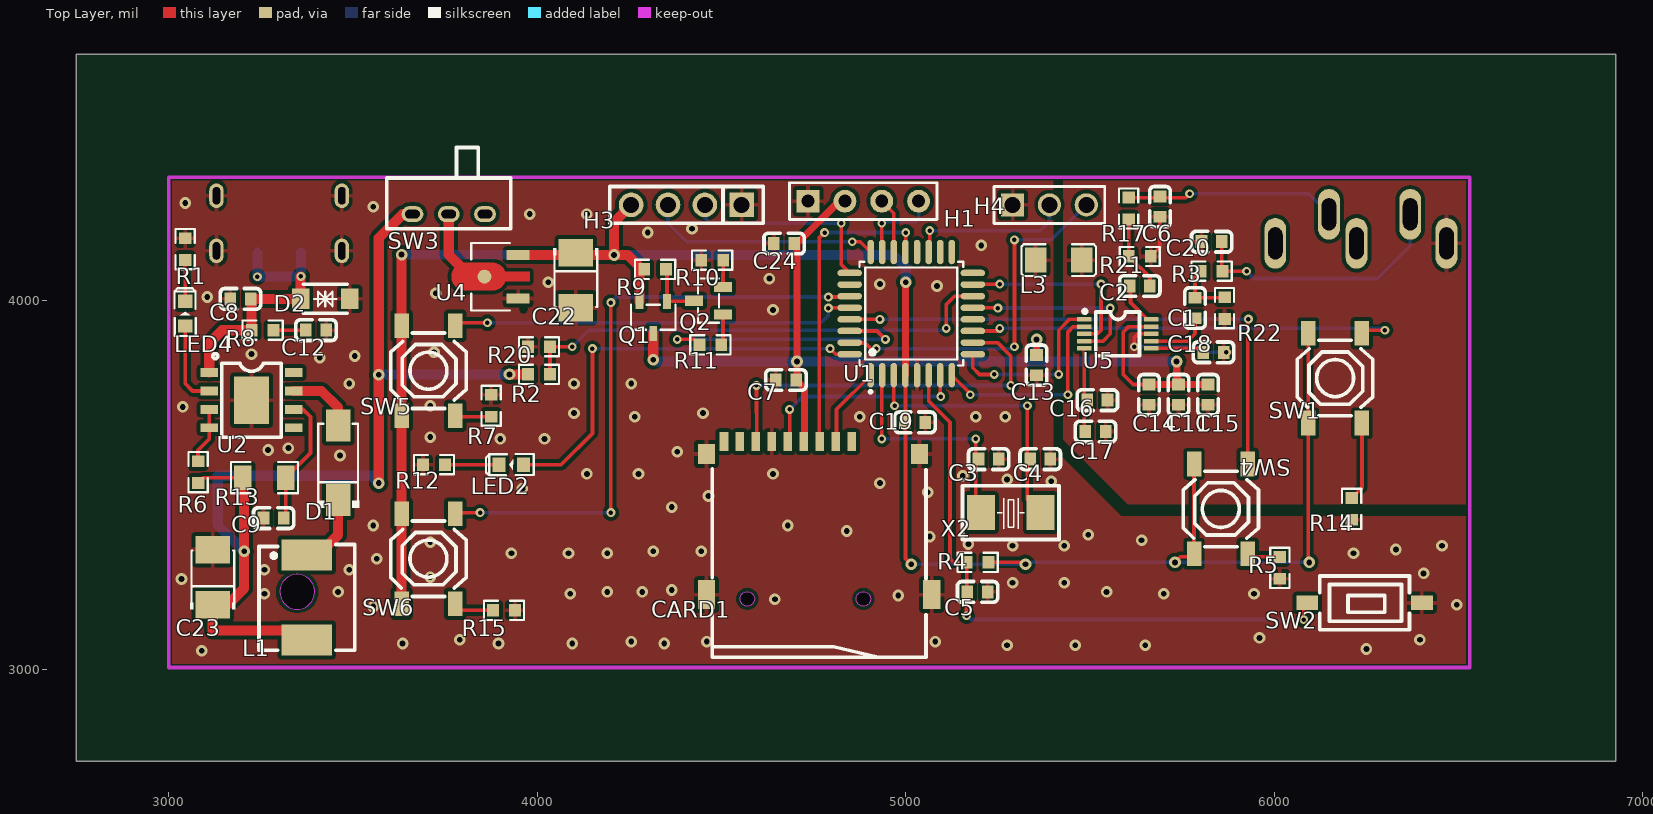
[diagram p0: Top Layer view]
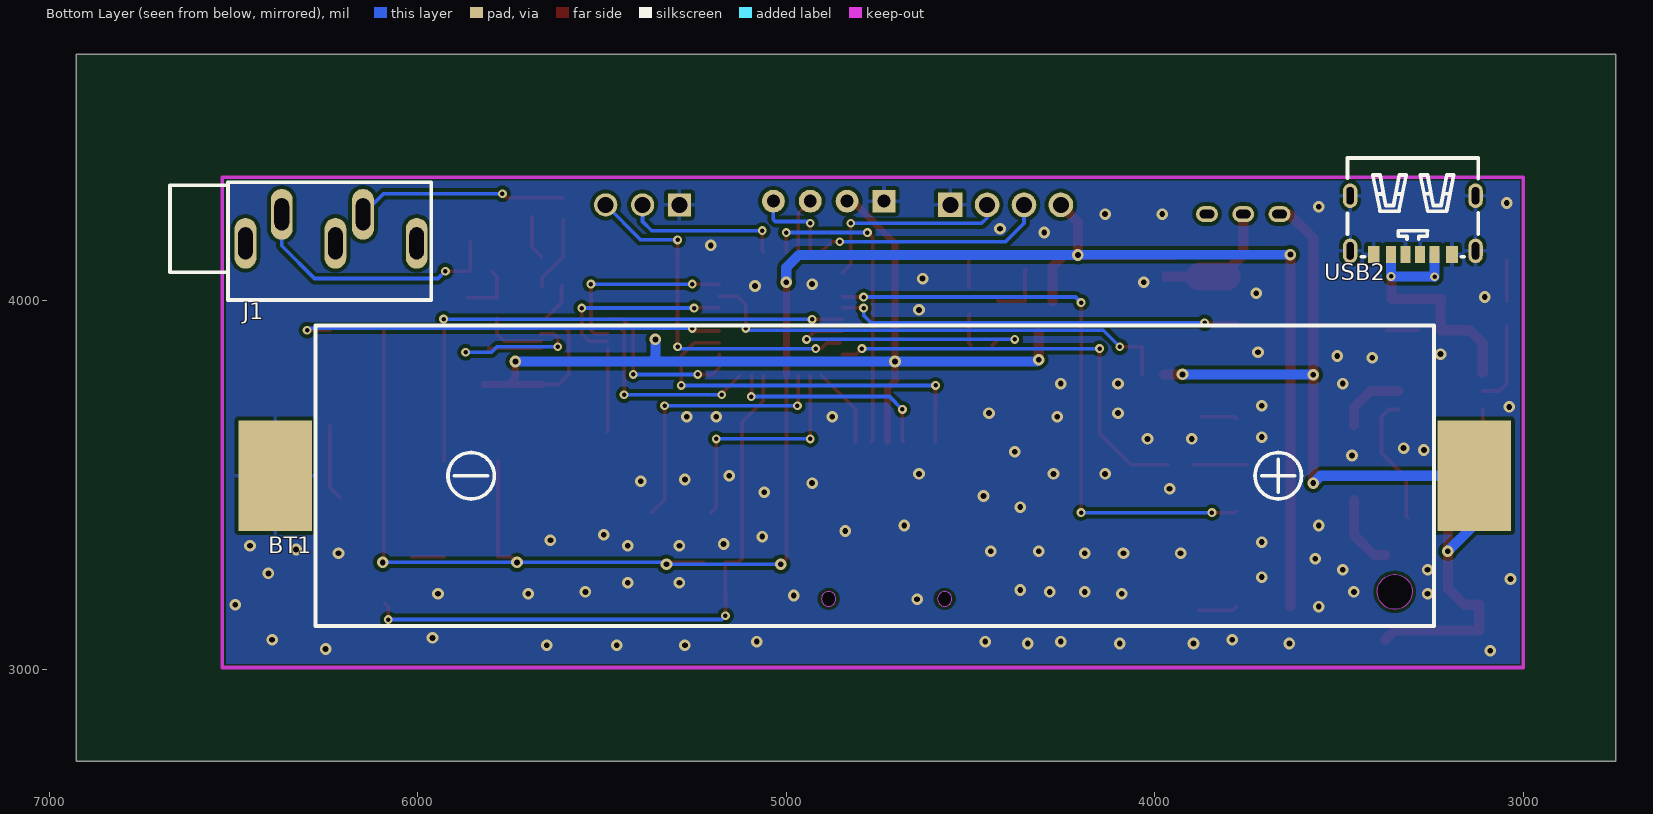
[diagram p1: Bottom Layer view, seen from below]
# Altium PCB MISC82317.pcbdoc
Units mil, origin at the board's own origin, x right, y up, seen from the top; angles counter-clockwise.
Board outline 4175.9 x 1918.1 mil, 2 copper layers (Top Layer, Bottom Layer), stack 62.2 mil thick; 67 components, 58 nets, 218 pads, 165 vias.

## Layer stack, top to bottom
Top Solder Mask Layer: solder mask 0.4, Dk 3.3
Top Layer: signal copper 1.4
Dielectric1: surface 59.4, FR4, Dk 4.5
Bottom Layer: signal copper 1.4
Bottom Solder Mask Layer: solder mask 0.4, Dk 3.3

## Board outline
6925.9,2750 2750,2750 2750,4668.1 6925.9,4668.1

## Design rules (kind name [scope] priority, off if disabled: settings)
BoardOutlineClearance copperThickness1oz [All] p0: genericclearance=10 ignorepadtopadclearanceinfootprint=FALSE except(0: Arc-SplitContinuation Track-SplitContinuation SMDPad-SplitContinuation THPad-SplitContinuation Via-SplitContinuation Fill-SplitContinuation Poly-SplitContinuation Region-SplitContinuation Text-SplitContinuation)
BoardOutlineClearance copperThickness2oz [All] p0: genericclearance=10 ignorepadtopadclearanceinfootprint=FALSE except(0: Arc-SplitContinuation Track-SplitContinuation SMDPad-SplitContinuation THPad-SplitContinuation Via-SplitContinuation Fill-SplitContinuation Poly-SplitContinuation Region-SplitContinuation Text-SplitContinuation)
BoardOutlineClearance otherClearance [All] p0: genericclearance=10 ignorepadtopadclearanceinfootprint=FALSE except(0: Arc-SplitContinuation Track-SplitContinuation SMDPad-SplitContinuation THPad-SplitContinuation Via-SplitContinuation Fill-SplitContinuation Poly-SplitContinuation Region-SplitContinuation Text-SplitContinuation)
Clearance copperThickness1oz [All] p1: gap=7 ignorepadtopadclearanceinfootprint=FALSE
Clearance copperThickness2oz [All] p1: gap=7 ignorepadtopadclearanceinfootprint=FALSE
Clearance otherClearance [All] p1: gap=7 ignorepadtopadclearanceinfootprint=FALSE
DiffPairsRouting differentialPair [All] p1: maxuncoupledlength=10 minlimit=6 maxlimit=Infinity mostfreqgap=6 toplayer_minwidth=5 toplayer_prefwidth=10 toplayer_maxwidth=100 bottomlayer_minwidth=5 bottomlayer_prefwidth=10 bottomlayer_maxwidth=100
PasteMaskExpansion pasteMaskExpansion [All] p1: expansion=0
PlaneConnect innerPlane [All] p1: planeconnectstyle=Relief reliefexpansion=20 reliefentries=4 reliefconductorwidth=10 reliefairgap=10
PolygonConnect copperRegion [All] p1: connectstyle=Relief reliefentries=4 reliefconductorwidth=10 polygonreliefangle="90 Angle" airgapwidth=10
RoutingVias viaSize [All] p1: viastyle="Through Hole" holewidth=12.0078 minholewidth=11.811 maxholewidth=248.0314 width=12.0078 minwidth=11.811 maxwidth=248.0314
SolderMaskExpansion solderMaskExpansion [IsVia] p1: useseparateexpansions=TRUE expansion=-1000 expansionbottom=-1000
SolderMaskExpansion solderMaskExpansion [All] p2: useseparateexpansions=TRUE expansion=2 expansionbottom=2
Width copperThickness1oz [All] p1: maxlimit=100 minlimit=5 preferedwidth=10
Width copperThickness2oz [All] p1: maxlimit=100 minlimit=8 preferedwidth=10

## Components (designator, comment, footprint, x,y, rotation, side; value= is the part's Value field where it differs from the comment)
BT1 "BH-18650-B1BA002" BATTERY-SMD_18650-1S-L77.1-W20.7-1 4760,3525 r270 bottom
C1 "2.2uF" C0603 5785,3980 r90 top
C2 "2.2uF" C0603 5635,4040 r0 top
C3 "20p" C0603 5225,3570 r180 top
C4 "20p" C0603 5365,3570 r180 top
C5 "10u" C0603 5195,3210 r180 top
C6 "2.2nf" C0603 5690,4255 r90 top
C7 "0.1uf" C0603 4675,3785 r0 top
C8 "22uf" C0603 3195,4005 r0 top
C9 "22uF" C0603 3285,3410 r0 top
C11 "0.1u" C0603 5740,3745 r90 top
C12 "10uF" C0603 3400,3920 r180 top
C13 "10u" C0603 5355,3825 r90 top
C14 "2.2uf" C0603 5660,3745 r90 top
C15 "10nf" C0603 5820,3745 r90 top
C16 "0.1u" C0603 5520,3730 r180 top
C17 "10u" C0603 5515,3645 r180 top
C18 "10u" C0603 5835,3860 r180 top
C19 "2.2uf" C0603 5025,3670 r180 top
C20 "2.2nf" C0603 5830,4160 r180 top
C22 "22uF" CAP-SMD_L3.5-W2.8-R-RD#1 4105,4055 r90 top
C23 "22uF" CAP-SMD_L3.5-W2.8-R-RD#2 3120,3250 r270 top
C24 "0.1uf" C0603 4670,4155 r0 top
CARD1 "TF-01A" TF-SMD_TF-01A 4765,3410 r0 top
D1 "SS14" SMA_L4.2-W2.6-LS5.3-RD 3460,3560 r90 top
D2 "SMF6.0CA" SOD-123FL_L2.8-W1.8-LS3.7-BI 3425,4005 r180 top
H1 "HDR-F-2.54_1x4" HDR-F-2.54_1X4 4885,4270 r0 top
H3 "220S-1*4P H=8.5MM" HDR-TH_4P-P2.54-V-F 4405,4260 r180 top
H4 "Z-211-0311-0021-001" HDR-TH_3P-P2.54-V-M-1 5390,4260 r0 top
J1 "PJ-325M/3.5MM" AUDIO-TH_PJ-325C 6235,4195 r180 bottom
L1 "1uH" IND-SMD_L6.8-W6.8_SMMS0630 3375,3195 r270 top
L3 "600Ω" L1206 5415,4110 r180 top
LED2 "LED-0603_G" LED0603_GREEN 3930,3555 r180 top
LED4 "LED-0603_G" LED0603_GREEN 3045,3965 r90 top
Q1 "SI2301CDS-T1-GE3" SOT-23-3_L3.0-W1.7-P0.95-LS2.9-BR 4315,3955 r90 top
Q2 "SI2302_C351401" SOT-23-3_L2.9-W1.3-P1.90-LS2.4 4465,3999.9 r0 top
R1 "10k" R0603 3045,4140 r90 top
R2 "47k" R0603 4005,3800 r180 top
R3 "470R" R0603 5830,4080 r180 top
R4 "1k" R0603 5195,3290 r0 top
R5 "10K" R0603 6015,3275 r90 top
R6 "120" R0603 3080,3535 r270 top
R7 "10K" R0603 3875,3715 r270 top
R8 "120" R0603 3255,3920 r0 top
R9 "1M" R0603 4320,4085 r0 top
R10 "100K" R0603 4475,4110 r180 top
R11 "10K" R0603 4470,3880 r0 top
R12 "10k" R0603 3720,3555 r0 top
R13 "0R5" R1206 3260,3520 r180 top
R14 "10K" R0603 6210,3435 r90 top
R15 "10K" R0603 3910,3160 r180 top
R17 "470R" R0603 5605,4250 r270 top
R20 "100k" R0603 4005,3875 r0 top
R21 "NA" R0603 5635,4120 r0 top
R22 "NA" R0603 5865,3980 r90 top
SW1 "TS-1187A-B-A-B" SW-SMD_4P-L5.1-W5.1-P3.70-LS6.5-TL-2 6165,3790 r90 top
SW2 "TS-1092S-B3D2-G" SW-SMD_L6.1-W3.6-LS7.9 6245,3180 r180 top
SW3 "MK-12D18-G020" SW-TH_MK-12D18-G040 3760,4235 r180 top
SW4 "TS-1187A-B-A-B" SW-SMD_4P-L5.1-W5.1-P3.70-LS6.5-TL-2 5855,3435 r90 top
SW5 "TS-1187A-B-A-B" SW-SMD_4P-L5.1-W5.1-P3.70-LS6.5-TL-2 3705,3810 r90 top
SW6 "TS-1187A-B-A-B" SW-SMD_4P-L5.1-W5.1-P3.70-LS6.5-TL-2 3705,3300 r90 top
U1 "STM32G070KBT6" LQFP-32_L7.0-W7.0-P0.80-LS9.0-BL 5015,3965 r0 top
U2 "IP5306" ESOP-8_L4.9-W3.9-P1.27-LS6.0-BL-EP 3225,3730 r270 top
U4 "HT7833" SOT-89_L4.5-W2.5-P1.50-LS4.2-BR 3895,4065 r0 top
U5 "CS4344" TSSOP-10_L3.0-W3.0-P0.50-LS4.9-BL 5575,3910 r270 top
USB2 "TYPE-C 6P" TYPE-C-SMD_TYPE-C-6P 3300,4205 r0 bottom
X2 "8MHz" CRYSTAL-SMD_L5.0-W3.2 5285,3425 r0 top

## Footprints (in the part's own frame and the unit in brackets; to place one, negate y for a bottom-side part, rotate by r counter-clockwise, add the part's x,y. Pads: shape width x height; smd on the part's side, far side on the other; paste and mask are expansions set on the pad)
AUDIO-TH_PJ-325C [mil]
  oval 59.1x137.8 hole 39.4 slot 86.6 at 90 deg: 1(-232.3,-39.4) 2(11.8,-39.4) 3(86.6,39.4) 4(232.3,-39.4) 5(-133.9,39.4)
  silkscreen extent -437,-193 272,126
BATTERY-SMD_18650-1S-L77.1-W20.7-1 [mil]
  rect 300x200 smd: 1(0,-1626.5) 2(0,1626.5)
  Board Outline Layer lines w0.1: 316.5,1458.2 310.4,1458 304.4,1457.1 298.6,1455.4 293.1,1452.9 287.9,1449.8 283.2,1446 279,1441.6 275.4,1436.8 272.4,1431.5 270.1,1425.9 268.6,1420.1 267.8,1414 267.8,1408 268.6,1402 270.1,1396.1 272.4,1390.5 275.4,1385.2 279,1380.4 283.2,1376 287.9,1372.3 293.1,1369.1 298.6,1366.7 304.4,1365 310.4,1364 316.5,1363.8 322.5,1364.4 328.4,1365.7 334.1,1367.8 339.5,1370.6 344.4,1374.1 348.9,1378.2 352.8,1382.8 356.1,1387.8 358.8,1393.3 360.7,1399 361.8,1405 362.2,1411 361.8,1417.1 360.7,1423 358.8,1428.7 356.1,1434.2 352.8,1439.3 348.9,1443.9 344.4,1448 339.5,1451.4 334.1,1454.2 328.4,1456.3 322.5,1457.7 316.5,1458.2
  Board Outline Layer region: 362.2,1411 361.8,1405 360.7,1399 358.8,1393.3 356.1,1387.8 352.8,1382.8 348.9,1378.2 344.4,1374.1 339.5,1370.6 334.1,1367.8 328.4,1365.7 322.5,1364.4 316.5,1363.8 310.4,1364 304.4,1365 298.6,1366.7 293.1,1369.1 287.9,1372.3 283.2,1376 279,1380.4 275.4,1385.2 272.4,1390.5 270.1,1396.1 268.6,1402 267.8,1408 267.8,1414 268.6,1420.1 270.1,1425.9 272.4,1431.5 275.4,1436.8 279,1441.6 283.2,1446 287.9,1449.8 293.1,1452.9 298.6,1455.4 304.4,1457.1 310.4,1458 316.5,1458.2 322.5,1457.7 328.4,1456.3 334.1,1454.2 339.5,1451.4 344.4,1448 348.9,1443.9 352.8,1439.3 356.1,1434.2 358.8,1428.7 360.7,1423 361.8,1417.1
  Board Outline Layer region: 362.2,1411 361.8,1405 360.7,1399 358.8,1393.3 356.1,1387.8 352.8,1382.8 348.9,1378.2 344.4,1374.1 339.5,1370.6 334.1,1367.8 328.4,1365.7 322.5,1364.4 316.5,1363.8 310.4,1364 304.4,1365 298.6,1366.7 293.1,1369.1 287.9,1372.3 283.2,1376 279,1380.4 275.4,1385.2 272.4,1390.5 270.1,1396.1 268.6,1402 267.8,1408 267.8,1414 268.6,1420.1 270.1,1425.9 272.4,1431.5 275.4,1436.8 279,1441.6 283.2,1446 287.9,1449.8 293.1,1452.9 298.6,1455.4 304.4,1457.1 310.4,1458 316.5,1458.2 322.5,1457.7 328.4,1456.3 334.1,1454.2 339.5,1451.4 344.4,1448 348.9,1443.9 352.8,1439.3 356.1,1434.2 358.8,1428.7 360.7,1423 361.8,1417.1
  Multi-Layer board cut-out: 362.2,1411 361.8,1405 360.7,1399 358.8,1393.3 356.1,1387.8 352.8,1382.8 348.9,1378.2 344.4,1374.1 339.5,1370.6 334.1,1367.8 328.4,1365.7 322.5,1364.4 316.5,1363.8 310.4,1364 304.4,1365 298.6,1366.7 293.1,1369.1 287.9,1372.3 283.2,1376 279,1380.4 275.4,1385.2 272.4,1390.5 270.1,1396.1 268.6,1402 267.8,1408 267.8,1414 268.6,1420.1 270.1,1425.9 272.4,1431.5 275.4,1436.8 279,1441.6 283.2,1446 287.9,1449.8 293.1,1452.9 298.6,1455.4 304.4,1457.1 310.4,1458 316.5,1458.2 322.5,1457.7 328.4,1456.3 334.1,1454.2 339.5,1451.4 344.4,1448 348.9,1443.9 352.8,1439.3 356.1,1434.2 358.8,1428.7 360.7,1423 361.8,1417.1
  silkscreen extent -408,-1518 408,1518
C0603 [mil]
  rect 31.5x35.4 smd: 1(-27.6,0) 2(27.6,0)
  silkscreen extent -55,-28 55,28
CAP-SMD_L3.5-W2.8-R-RD#1 [mil]
  rect 74.8x93.5 smd: 1(74.8,0) 2(-74.7,0)
  silkscreen extent -72,-61 87,61
CAP-SMD_L3.5-W2.8-R-RD#2 [mil]
  rect 74.8x93.5 smd: 1(74.7,0) 2(-74.8,0)
  silkscreen extent -72,-61 87,61
CRYSTAL-SMD_L5.0-W3.2 [mil]
  rect 74.8x94.5 smd: 1(-80.7,0) 2(80.7,0)
  silkscreen extent -131,-73 131,73
ESOP-8_L4.9-W3.9-P1.27-LS6.0-BL-EP [mil]
  rect 23.6x47.2 smd: 1(-75,-114.5) 2(-25,-114.5) 3(25,-114.5) 4(75,-114.5) 5(75,114.5) 6(25,114.5) 7(-25,114.5) 8(-75,114.5)
  rect 129.9x94.5 smd: 9(0,0)
  silkscreen extent -126,-105 100,81
HDR-F-2.54_1X4 [mil]
  rect 62x62 hole 35: 1(-150,0)
  round 62 hole 35: 2(-50,0) 3(50,0) 4(150,0)
  silkscreen extent -200,-50 200,50
HDR-TH_3P-P2.54-V-M-1 [mil]
  rect 62x63 hole 43.3 paste+0 mask+2: 1(-100,0)
  round 63 hole 43.3 paste+0 mask+2: 2(0,0) 3(100,0)
  silkscreen extent -150,-50 150,50
HDR-TH_4P-P2.54-V-F [mil]
  rect 66.9x66.9 hole 43.3: 1(-150,0)
  round 66.9 hole 43.3: 2(-50,0) 3(50,0) 4(150,0)
  silkscreen extent -208,-50 208,50
IND-SMD_L6.8-W6.8_SMMS0630 [mil]
  rect 84.6x137.8 smd paste+0 mask+2: 1(-115.2,0) 2(115.2,0)
  silkscreen extent -144,-130 144,130
L1206 [mil]
  rect 58.5x68 smd paste-3937 mask+2: 1(-62.7,0) 2(62.7,0)
  silkscreen extent -101,-43 101,43
LED0603_GREEN [mil]
  rect 35.4x39.4 smd: 1(-33.5,0) 2(33.5,0)
  silkscreen extent -61,-29 69,29
LQFP-32_L7.0-W7.0-P0.80-LS9.0-BL [mil]
  oval 17.6x66.3 smd: 1(-110.2,-167) 2(-78.7,-167) 3(-47.2,-167) 4(-15.7,-167) 5(15.8,-167) 6(47.2,-167) 7(78.7,-167) 8(110.2,-167) 17(110.2,167) 18(78.7,167) 19(47.2,167) 20(15.8,167) 21(-15.7,167) 22(-47.2,167) 23(-78.7,167) 24(-110.2,167)
  oval 66.3x17.6 smd: 9(167,-110.2) 10(167,-78.7) 11(167,-47.2) 12(167,-15.7) 13(167,15.8) 14(167,47.2) 15(167,78.7) 16(167,110.2) 25(-167,110.2) 26(-167,78.7) 27(-167,47.2) 28(-167,15.8) 29(-167,-15.7) 30(-167,-47.2) 31(-167,-78.7) 32(-167,-110.2)
  silkscreen extent -141,-216 141,141
R0603 [mil]
  rect 31.8x34 smd paste-3937 mask+2: 1(-29.7,0) 2(29.7,0)
  silkscreen extent -54,-26 54,26
R1206 [mil]
  rect 47.5x67 smd paste-3937 mask+2: 1(-58.2,0) 2(58.2,0)
  silkscreen extent -91,-43 91,43
SMA_L4.2-W2.6-LS5.3-RD [mil]
  rect 86.6x66.9 smd: 1(-101,0) 2(101,0)
  silkscreen extent -121,-57 106,57
SOD-123FL_L2.8-W1.8-LS3.7-BI [mil]
  rect 47.2x55.1 smd: 1(-66.9,0) 2(66.9,0)
  silkscreen extent -59,-39 59,39
SOT-23-3_L2.9-W1.3-P1.90-LS2.4 [mil]
  rect 49.2x27.6 smd: 1(39.4,-37.4) 2(39.4,37.4) 3(-39.3,0)
  silkscreen extent -28,-60 29,60
SOT-23-3_L3.0-W1.7-P0.95-LS2.9-BR [mil]
  rect 40.8x20.9 smd: 1(43.4,-37.4) 2(43.4,37.4) 3(-43.4,0)
  silkscreen extent -34,-60 34,60
SOT-89_L4.5-W2.5-P1.50-LS4.2-BR [mil]
  rect 62x26.5 smd paste+0 mask+2: 1(53.4,-59.1) 3(53.4,59.1)
  round 37.4 smd: 2(-38,0.3)
  Top Layer region: -89.9,37.7 -16.9,37.7 -15.1,37.7 -13.4,37.6 -11.6,37.4 -9.9,37.1 -8.2,36.7 -6.5,36.3 -4.8,35.7 -3.2,35.1 -1.6,34.5 0,33.7 1.6,32.9 3.1,32 4.5,31 5.9,30 7.3,28.9 8.6,27.7 9.9,26.5 11.1,25.2 12.2,23.9 13.3,22.5 14.3,21 15.2,19.5 16.1,18 16.9,16.5 17.6,13.3 84.4,13.3 84.4,-12.6 17.6,-12.6 16.9,-15.8 16.1,-17.3 15.2,-18.9 14.3,-20.3 13.3,-21.8 12.2,-23.2 11.1,-24.5 9.9,-25.8 8.6,-27 7.3,-28.2 5.9,-29.3 4.5,-30.3 3.1,-31.3 1.6,-32.2 0,-33 -1.6,-33.8 -3.2,-34.5 -4.8,-35.1 -6.5,-35.6 -8.2,-36 -9.9,-36.4 -11.6,-36.7 -13.4,-36.9 -15.1,-37 -16.9,-37.1 -89.9,-37.1 -91.6,-37 -93.4,-36.9 -95.1,-36.7 -96.9,-36.4 -98.6,-36 -100.3,-35.6 -101.9,-35.1 -103.6,-34.5 -105.2,-33.8 -106.8,-33 -108.3,-32.2 -109.8,-31.3 -111.3,-30.3 -112.7,-29.3 -114.1,-28.2 -115.4,-27 -116.6,-25.8 -117.8,-24.5 -119,-23.2 -120,-21.8 -121.1,-20.3 -122,-18.9 -122.8,-17.3 -123.6,-15.8 -124.4,-14.2 -125,-12.5 -125.6,-10.9 -126.1,-9.2 -126.5,-7.5 -126.8,-5.8 -127,-4 -127.2,-2.3 -127.3,-0.5 -127.3,1.2 -127.2,3 -127,4.7 -126.8,6.5 -126.5,8.2 -126.1,9.9 -125.6,11.6 -125,13.2 -124.4,14.9 -123.6,16.5 -122.8,18 -122,19.5 -121.1,21 -120,22.5 -119,23.9 -117.8,25.2 -116.6,26.5 -115.4,27.7 -114.1,28.9 -112.7,30 -111.3,31 -109.8,32 -108.3,32.9 -106.8,33.7 -105.2,34.5 -103.6,35.1 -101.9,35.7 -100.3,36.3 -98.6,36.7 -96.9,37.1 -95.1,37.4 -93.4,37.6 -91.6,37.7
  silkscreen extent -74,-92 31,92
SW-SMD_4P-L5.1-W5.1-P3.70-LS6.5-TL-2 [mil]
  rect 66.9x39.4 smd: 1(-122,72.8) 2(122,72.8) 3(-122,-72.8) 4(122,-72.8)
  silkscreen extent -102,-102 102,102
SW-SMD_L6.1-W3.6-LS7.9 [mil]
  rect 59.1x39.4 smd: 1(-155.5,0) 2(155.5,0)
  silkscreen extent -122,-73 122,73
SW-TH_MK-12D18-G040 [mil]
  oval 59.1x43.3 hole 23.6 slot 39.4 at 0 deg paste+0 mask+2: 1(-98.4,0) 2(0,0) 3(98.4,0)
  silkscreen extent -168,-181 168,40
TF-SMD_TF-01A [mil]
  rect 23.6x51.2 smd: 1(88.2,207.7) 2(44.9,207.7) 3(1.6,207.7) 4(-41.7,207.7) 5(-85,207.7) 6(-128.3,207.7) 7(-171.7,207.7) 8(-215,207.7) 9(-258.3,207.7)
  rect 47.2x55.1 smd: 10(-305.5,174.2) 13(272.4,174.2)
  rect 47.2x78.7 smd: 11(-305.5,-207.7) 12(305.5,-207.7)
  Board Outline Layer lines w0.1: -214.6,-219.1 -214.2,-223 -213.1,-226.7 -211.2,-230.1 -208.8,-233.1 -205.8,-235.5 -202.4,-237.3 -198.7,-238.4 -194.9,-238.8 -191,-238.4 -187.3,-237.3 -183.9,-235.5 -181,-233.1 -178.5,-230.1 -176.7,-226.7 -175.6,-223 -175.2,-219.1 -175.6,-215.3 -176.7,-211.6 -178.5,-208.2 -181,-205.2 -183.9,-202.8 -187.3,-201 -191,-199.8 -194.9,-199.5 -198.7,-199.8 -202.4,-201 -205.8,-202.8 -208.8,-205.2 -211.2,-208.2 -213.1,-211.6 -214.2,-215.3 -214.6,-219.1 ; 100.4,-219.1 100.8,-223 101.9,-226.7 103.7,-230.1 106.2,-233.1 109.1,-235.5 112.5,-237.3 116.2,-238.4 120.1,-238.8 123.9,-238.4 127.6,-237.3 131,-235.5 134,-233.1 136.4,-230.1 138.3,-226.7 139.4,-223 139.8,-219.1 139.4,-215.3 138.3,-211.6 136.4,-208.2 134,-205.2 131,-202.8 127.6,-201 123.9,-199.8 120.1,-199.5 116.2,-199.8 112.5,-201 109.1,-202.8 106.2,-205.2 103.7,-208.2 101.9,-211.6 100.8,-215.3 100.4,-219.1
  Board Outline Layer region: -175.2,-219.1 -175.6,-223 -176.7,-226.7 -178.5,-230.1 -181,-233.1 -183.9,-235.5 -187.3,-237.3 -191,-238.4 -194.9,-238.8 -198.7,-238.4 -202.4,-237.3 -205.8,-235.5 -208.8,-233.1 -211.2,-230.1 -213.1,-226.7 -214.2,-223 -214.6,-219.1 -214.2,-215.3 -213.1,-211.6 -211.2,-208.2 -208.8,-205.2 -205.8,-202.8 -202.4,-201 -198.7,-199.8 -194.9,-199.5 -191,-199.8 -187.3,-201 -183.9,-202.8 -181,-205.2 -178.5,-208.2 -176.7,-211.6 -175.6,-215.3
  Board Outline Layer region: -175.2,-219.1 -175.6,-223 -176.7,-226.7 -178.5,-230.1 -181,-233.1 -183.9,-235.5 -187.3,-237.3 -191,-238.4 -194.9,-238.8 -198.7,-238.4 -202.4,-237.3 -205.8,-235.5 -208.8,-233.1 -211.2,-230.1 -213.1,-226.7 -214.2,-223 -214.6,-219.1 -214.2,-215.3 -213.1,-211.6 -211.2,-208.2 -208.8,-205.2 -205.8,-202.8 -202.4,-201 -198.7,-199.8 -194.9,-199.5 -191,-199.8 -187.3,-201 -183.9,-202.8 -181,-205.2 -178.5,-208.2 -176.7,-211.6 -175.6,-215.3
  Board Outline Layer region: 139.8,-219.1 139.4,-223 138.3,-226.7 136.4,-230.1 134,-233.1 131,-235.5 127.6,-237.3 123.9,-238.4 120.1,-238.8 116.2,-238.4 112.5,-237.3 109.1,-235.5 106.2,-233.1 103.7,-230.1 101.9,-226.7 100.8,-223 100.4,-219.1 100.8,-215.3 101.9,-211.6 103.7,-208.2 106.2,-205.2 109.1,-202.8 112.5,-201 116.2,-199.8 120.1,-199.5 123.9,-199.8 127.6,-201 131,-202.8 134,-205.2 136.4,-208.2 138.3,-211.6 139.4,-215.3
  Board Outline Layer region: 139.8,-219.1 139.4,-223 138.3,-226.7 136.4,-230.1 134,-233.1 131,-235.5 127.6,-237.3 123.9,-238.4 120.1,-238.8 116.2,-238.4 112.5,-237.3 109.1,-235.5 106.2,-233.1 103.7,-230.1 101.9,-226.7 100.8,-223 100.4,-219.1 100.8,-215.3 101.9,-211.6 103.7,-208.2 106.2,-205.2 109.1,-202.8 112.5,-201 116.2,-199.8 120.1,-199.5 123.9,-199.8 127.6,-201 131,-202.8 134,-205.2 136.4,-208.2 138.3,-211.6 139.4,-215.3
  Multi-Layer board cut-out: -175.2,-219.1 -175.6,-223 -176.7,-226.7 -178.5,-230.1 -181,-233.1 -183.9,-235.5 -187.3,-237.3 -191,-238.4 -194.9,-238.8 -198.7,-238.4 -202.4,-237.3 -205.8,-235.5 -208.8,-233.1 -211.2,-230.1 -213.1,-226.7 -214.2,-223 -214.6,-219.1 -214.2,-215.3 -213.1,-211.6 -211.2,-208.2 -208.8,-205.2 -205.8,-202.8 -202.4,-201 -198.7,-199.8 -194.9,-199.5 -191,-199.8 -187.3,-201 -183.9,-202.8 -181,-205.2 -178.5,-208.2 -176.7,-211.6 -175.6,-215.3
  Multi-Layer board cut-out: 139.8,-219.1 139.4,-223 138.3,-226.7 136.4,-230.1 134,-233.1 131,-235.5 127.6,-237.3 123.9,-238.4 120.1,-238.8 116.2,-238.4 112.5,-237.3 109.1,-235.5 106.2,-233.1 103.7,-230.1 101.9,-226.7 100.8,-223 100.4,-219.1 100.8,-215.3 101.9,-211.6 103.7,-208.2 106.2,-205.2 109.1,-202.8 112.5,-201 116.2,-199.8 120.1,-199.5 123.9,-199.8 127.6,-201 131,-202.8 134,-205.2 136.4,-208.2 138.3,-211.6 139.4,-215.3
  silkscreen extent -290,-377 290,134
TSSOP-10_L3.0-W3.0-P0.50-LS4.9-BL [mil]
  rect 11.8x39.4 smd: 1(-39.4,-90.6) 2(-19.7,-90.6) 3(0,-90.6) 4(19.7,-90.6) 5(39.4,-90.6) 6(39.4,90.6) 7(19.7,90.6) 8(0,90.6) 9(-19.7,90.6) 10(-39.4,90.6)
  silkscreen extent -66,-94 59,59
TYPE-C-SMD_TYPE-C-6P [mil]
  oval 39.4x66.9 hole 19.7 slot 47.2 at 90 deg paste+0 mask+2: 7(-170.1,-79.7) 7(-170.1,69.9) 7(170.1,-79.7) 7(170.1,69.9)
  rect 27.6x47.2 smd paste+0 mask+2: A5(-19.7,79.7) A9(59,79.7) B5(19.7,79.7) B9(-59.1,79.7)
  rect 31.5x47.2 smd paste+0 mask+2: A12(106.3,79.7) B12(-106.3,79.7)
  silkscreen extent -177,-182 177,86

## Via types
v1: diameter 31.5, hole 15.7, Top Layer to Bottom Layer, 116 vias
v2: diameter 24, hole 12.2, Top Layer to Bottom Layer, 47 vias
v3: diameter 24, hole 12, Top Layer to Bottom Layer, 2 vias

## Nets (pads, with @x,y where several pads share a name; then routed paths per layer and width w, separated by ;. In a path a pad name is that pad's centre, name@x,y a point inside that pad or via, vN(x,y) a via of type N, cw(c..) or ccw(c..) an arc to the next point about the centre after c; other vN are vias at no path point)
$1N1: R15.2 SW6.3 | length 106.7
  Top Layer w10: SW6.3@3777.8,3170.1 3787.9,3160 R15.2
$1N3: R7.2 SW5.3 | length 99.3
  Top Layer w10: SW5.3@3777.8,3680.1 3783.1,3685.3 R7.2
$1N5: R5.2 SW4.3 | length 87.1
  Top Layer w10: SW4.3@5927.9,3305.1 R5.2
$1N10: LED4.2 R1.1 | length 111.8
  Top Layer w10: LED4.2 R1.1
$1N24: R14.2 SW1.3 | length 207
  Top Layer w10: R14.2 6237.9,3492.5 SW1.3@6237.9,3660.1
$1N27: LED2.2 R12.2 | length 146.8
  Top Layer w10: R12.2 LED2.2
$1N29: Q2.2 R10.1 | length 72.6
  Top Layer w10: Q2.2@4504.4,4037.4 R10.1
$1N30: Q2.1 R11.2 | length 84.5
  Top Layer w10: R11.2 4504.4,3884.8 Q2.1@4504.4,3962.6
$1N54: C12.2 R8.2 | length 87.7
  Top Layer w10: R8.2 C12.2
$1N57: D1.1 L1.1 | length 201.7
  Top Layer w27.6: L1.1 3405.2,3310.2 3460,3365 D1.1
$1N70: C1.2 R3.2 R22.2 | length 159.6
  Top Layer w10: R3.2 5785,4064.7 C1.2 5862.9,4007.6 R22.2
$1N71: C2.2 R17.2 R21.1 | length 204.2
  Top Layer w10: R17.2 5605.3,4220 R21.1 5662.6,4062.8 C2.2
$1N81: C18.2 U5.6 | length 152.4
  Top Layer w10: U5.6 5807.4,3870.6 C18.2
$1N104: C16.2 C17.2 U5.5 | length 226.8
  Top Layer w10: U5.5 5484.4,3648 C17.2
$1N113: Q1.1 Q2.3 R9.2 | length 161.6
  Top Layer w10: R9.2 4352.4,4082.3 Q1.1 4424.1,3998.4 Q2.3
$1N116: C9.2 R13.1 U2.6 | length 358.7
  Top Layer w10: C9.2 3318.2,3415.7 R13.1 3385,3586.8 3385,3685 3365,3705 U2.6
$1N117: D1.2 U2.7 | length 188.1
  Top Layer w27.6: U2.7 3415,3755 3460,3710 D1.2
$1N119: R6.1 U2.3 U2.4 | length 152.9
  Top Layer w10: R6.1 3080,3594.5 3110.5,3625 U2.4 U2.3
$1N120: SW3.2 U4.2 | length 216.3
  Top Layer w27.6: SW3.2 3760,4125 3819.7,4065.3 U4.2@3841.6,4065.3
$1N123: LED4.1 U2.2 | length 230.3
  Top Layer w10: LED4.1 3045,3775 3065,3755 U2.2
$1N128: C6.2 J1.3 R17.1 | length 570.7
  Top Layer w10: R17.1 5759.7,4279.7 v2(5770,4290)
  Bottom Layer w10: v2(5770,4290) 6092.8,4290 J1.3
$1N129: C20.1 J1.5 R3.1 | length 720.7
  Top Layer w10: C20.1 5857.6,4082.1 R3.1 v2(5925,4080)
  Bottom Layer w10: v2(5925,4080) 5945,4060 6280,4060 6368.9,4148.9 J1.5
A-GND: C6.1 C11.1 C14.1 C15.1 C16.1 C17.1 C18.1 C20.2 J1.1 L3.1 R21.2 R22.1 U5.8 | length 448.8
  Top Layer w10: v3(5620,3875) 5620,3900 5630,3910 U5.8 ; R21.2 5690,4145.3 C6.1
  Bottom Layer w10: v3(5620,3875) 5785,3875 5800,3860 v3(5870,3860)
AUDIO-L: C1.1 U5.7 | length 170
  Top Layer w10: U5.7 5765.3,3890.3 5785,3910 C1.1
AUDIO-R: C2.1 U5.10 | length 120.6
  Top Layer w10: C2.1 5610,4037.4 5610,3995 5655.6,3949.4 U5.10
BADC: R2.1 R20.2 U1.14 | length 1327.2
  Top Layer w10: R2.1 R20.2 v2(4095,3875) ; v2@5115,3920 v2(5110,3925) 5110,3990 5132.2,4012.2 U1.14
  Bottom Layer w10: v2(4095,3875) 4140,3920 5110,3920 v2(5110,3925)
GND: BT1.1 C3.1 C4.1 C5.1 C7.1 C8.1 C9.1 C12.1 C13.1 C19.1 C22.2 C23.2 C24.1 CARD1.6 CARD1.10 CARD1.11 CARD1.12 CARD1.13 D2.1 H1.1 H3.1 H4.1 L3.2 R1.2 R5.1 R7.1 R10.2 R12.1 R14.1 R15.1 R20.1 SW2.1 U1.5 U2.9 U4.1 USB2.7 USB2.A5 USB2.A12 USB2.B5 USB2.B12
  other v1: 3090,3050 6250,3055 5275,3065 5460,3065 5650,3065 3635,3070 3895,3070 4095,3070 4345,3070 4255,3075 4460,3075 5080,3075 3790,3080 6395,3080 5960,3085 3555,3170 6495,3175 4645,3190 4980,3200 3260,3205 4090,3205 5700,3205 5945,3205 3460,3210 4190,3210 4285,3210 5545,3210 4365,3215 5290,3235 5430,3235 3035,3245 3710,3250 6405,3260 3260,3270 3490,3270 3565,3300 3930,3315 4085,3315 4190,3315 6215,3315 4315,3320 4445,3320 6330,3325 5290,3335 5430,3335 6455,3335 5170,3340 3710,3345 5640,3350 5065,3360 5495,3365 4840,3375 3555,3390 4680,3390 4365,3440 4465,3470 5060,3480 3960,3490 4930,3505 5395,3510 5275,3515 5155,3525 4135,3530 4275,3530 4640,3530 3465,3580 4380,3590 3270,3595 3325,3600 3900,3625 4020,3625 3710,3630 4265,3685 4875,3685 5190,3685 5270,3685 4100,3695 4450,3695 3038.3,3711.8 3710,3715 3490,3775 4100,3775 4255,3775 3410,3845 3505,3850 3225,3855 3720,3860 4640,3975 3105,4010 3725,4020 5085,4040 4930,4045 4030,4050 4630,4060 5205,4150 4300,4185 4420,4195 3980,4235 4135,4235 3555,4255 3045,4265
I2S-CLK: U1.8 U5.2 | length 559.2
  Top Layer w10: U1.8 5175,3748.2 v2(5175,3745) ; v2(5440,3745) 5440,3915 5454.7,3929.7 U5.2@5484.5,3929.7
  Bottom Layer w10: v2(5175,3745) v2(5440,3745)
I2S-MCLK: U1.13 U5.4 | length 521.8
  Top Layer w10: U1.13@5182,3980.7 v2(5250,3980) ; U5.4 5535.3,3890.3 5555,3910 v2(5555,3980)
  Bottom Layer w10: v2(5250,3980) v2(5555,3980)
I2S-SDIN: U1.9 U5.1 | length 478.9
  Top Layer w10: U1.9 5182,3818 5200,3800 v2(5240,3800) ; v2(5415,3800) 5415,3920 5444.4,3949.4 U5.1@5484.5,3949.4
  Bottom Layer w10: v2(5240,3800) v2(5415,3800)
I2S-WS: U1.15 U5.3 | length 523.2
  Top Layer w10: U1.15 5183.3,4045 v2(5255,4045) ; U5.3@5484.5,3910 5520,3910 5530,3920 v2(5530,4045)
  Bottom Layer w10: v2(5255,4045) v2(5530,4045)
KEY-2:  | length 1468.2
  Top Layer w10: 4848,3949.3 v2(4930,3949.3) ; 5927.9,3564.9 5927.9,3947.8 v2(5930,3950)
  Bottom Layer w10: v2(4930,3949.3) 5929.3,3949.3 v2(5930,3950)
Key-2: SW4.4 U1.29
KEY-3:  | length 1098.5
  Top Layer w10: 3777.8,3939.9 v2(3865,3940) ; v2(4790,3980) 4848,3980.7
  Bottom Layer w10: v2(3865,3940) 4770,3940 4790,3960 v2(4790,3980)
Key-3: SW5.4 U1.28
KEY-4:  | length 1649.3
  Top Layer w10: 3777.8,3429.9 3782.8,3425 v2(3845,3425) ; v2(4200,3425) v2(4200,3995) ; v2(4790,4010) 4845.8,4010 4848,4012.2
  Bottom Layer w10: v2(3845,3425) v2(4200,3425) ; v2(4200,3995) 4215,4010 v2(4790,4010)
Key-4: SW6.4 U1.27
KEY-WAKE:  | length 1185.2
  Top Layer w10: 5182,3917.8 5247.8,3917.8 v2(5255,3925) ; 6237.9,3919.9 v2(6300,3920)
  Bottom Layer w10: v2(5255,3925) 6295,3925 v2(6300,3920)
Key-Wake: SW1.4 U1.11
NRST: C5.2 R4.1 SW2.2 U1.6 | length 1686.3
  Top Layer w10: U1.6 5062.2,3727.8 5120,3670 5120,3300 5130,3290 R4.1 5165.3,3212.1 C5.2 5165,3207.6 v2(5165,3145) ; v2(6080,3135) 6080,3170.5 SW2.2
  Bottom Layer w10: v2(5165,3145) 5175,3135 v2(6080,3135)
PERI-CNT: R11.1 U1.30 | length 738
  Top Layer w10: v2(4380,3895) 4425.3,3895 R11.1 ; U1.30 4922.2,3917.8 v2(4945,3895)
  Bottom Layer w10: v2(4380,3895) v2(4945,3895)
SCL: H1.3 U1.22 | length 151.6
  Top Layer w10: H1.3 4967.8,4237.2 U1.22
SDA: H1.4 U1.23 | length 235.6
  Top Layer w10: v2(4935,4210) 4935,4133.3 U1.23
  Bottom Layer w10: v2(4935,4210) 4935,4215 5030,4215 5035,4220 H1.4
SPI-CS: CARD1.2 U1.1 | length 218.6
  Top Layer w10: CARD1.2@4812.3,3617.7 4812.3,3705.5 U1.1
SPI-MISO: CARD1.7 U1.10 | length 1040.3
  Top Layer w10: v2(4595,3770) CARD1.7@4595.7,3617.7 ; U1.10 5248.7,3886.3 5285,3850 v2(5285,3770)
  Bottom Layer w10: v2(4595,3770) v2(5285,3770)
SPI-MOSI: CARD1.3 U1.21 | length 848.2
  Top Layer w10: CARD1.3@4769,3617.7 4765,3621.7 4765,4170 v2(4780,4185) ; U1.21 v2(5000,4185)
  Bottom Layer w10: v2(4780,4185) v2(5000,4185)
SPI-SCK: CARD1.5 U1.7 | length 571.4
  Top Layer w10: CARD1.5@4682.4,3617.7 4685,3620.4 v2(4685,3705) ; U1.7 5093.7,3741.3 v2(5095,3740)
  Bottom Layer w10: v2(4685,3705) 4720,3740 v2(5095,3740)
SWCLK: H3.2 U1.25 | length 555.5
  Top Layer w10: v2(4825,4210) 4825,4098.2 U1.25
  Bottom Layer w10: H3.2 4455,4225 4470,4210 v2(4825,4210)
SWDIO: H3.3 U1.24 | length 632.1
  Top Layer w10: v2(4855,4160) 4876.8,4160 U1.24
  Bottom Layer w10: H3.3 4355,4210 4405,4160 v2(4855,4160)
UART1_RX: H4.3 U1.31 | length 972.6
  Top Layer w10: U1.31@4855,3885 4890,3885 4905,3870 v2(4920,3870) ; v2(5295,3875) v2(5295,4165)
  Bottom Layer w10: v2(4920,3870) 5290,3870 v2(5295,3875) ; v2(5295,4165) 5395,4165 H4.3
UART1_TX: H4.2 U1.19 | length 439.5
  Top Layer w10: U1.19 5065,4134.8 v2(5065,4190)
  Bottom Layer w10: v2(5065,4190) 5365,4190 5390,4215 H4.2
VBAT: BT1.2 C23.1 L1.2 R2.2 R6.2 R13.2 SW3.3 | length 2736.6
  Top Layer w10: R6.2 3094.7,3520 R13.2
  Top Layer w27.6: R13.2 3205,3516.8 v1(3205,3320) 3205,3220 3160.2,3175.2 3120,3175.2 3120,3105 3349.8,3105 L1.2 ; v1(3570,3505) v1(3570,3799.2) 3570,4170 3635,4235 SW3.3 ; v1(3925,3800) R2.2
  Bottom Layer w27.6: v1(3205,3320) 3133.5,3391.5 BT1.2 3550,3525 v1(3570,3505) ; v1(3570,3799.2) v1(3925,3800)
VCC3.3: C19.2 C22.1 H3.4 Q1.2 R4.2 R9.1 SW1.1 SW1.2 SW4.1 SW4.2 SW5.1 SW5.2 SW6.1 SW6.2 U1.4 U4.3 | length 5873.1
  Top Layer w10: U1.4 4999.3,3300.7 v1(5015,3285) ; R4.2 5320,3290 v1(5325,3285) ; v1(5730.7,3290) 5745.8,3305.1 5782.2,3305.1 SW4.2@5782.1,3564.9 ; SW1.2@6092.1,3919.9 6092.2,3660.1 6092.2,3292.8 v1(6095,3290)
  Top Layer w19.7: U1.4 4999.3,4049.3 v1(5000,4050)
  Top Layer w27.6: SW6.1@3632.2,3170.1 3632.2,3939.9 v1(3632.2,4125) ; U4.3 v1(4208.7,4124.1) ; H3.4 4208.7,4213.7 v1(4208.7,4124.1) ; Q1.2 4277.6,4092.4 4245.9,4124.1 v1(4208.7,4124.1)
  Bottom Layer w10: v1(5015,3285) v1(5325,3285) 5330,3290 v1(5730.7,3290) v1(6095,3290)
  Bottom Layer w27.6: v1(3632.2,4125) v1(4208.7,4124.1) 4965.9,4124.1 5000,4090 v1(5000,4050)
VCC3.3-PERI: C7.2 C11.2 C13.2 C14.2 C15.2 C24.2 CARD1.4 H1.2 Q1.3 U5.9 | length 2814.6
  Top Layer w10: C14.2 5617.4,3772.6 5590,3800 5590,3915 5604.7,3929.7 U5.9
  Top Layer w19.7: CARD1.4@4725.6,3617.7 4725.6,3761.9 C7.2 4705,3787.4 v1(4705,3835) 4705,4155 4820,4270 H1.2 ; C13.2 v1(5355,3895) ; C14.2 C11.2 ; v1(5735,3835) 5735,3790 5752.4,3772.6 C15.2
  Top Layer w27.6: v1(4315,3840) Q1.3
  Bottom Layer w27.6: v1(4315,3840) 4320,3835 v1(4705,3835) v1(5735,3835) ; v1(5355,3895) 5355,3846.8 5361.8,3840
VCC5.0-USB: C8.2 D2.2 R8.1 U2.1 USB2.A9 USB2.B9 | length 739.9
  Top Layer w27.6: U2.1 3110.5,3884.5 3145,3920 R8.1 3225.3,4002.2 C8.2 D2.2 3358.1,4064.9 v2(3359.1,4065.9)
  Bottom Layer w27.6: USB2.B9@3240.9,4130.2 v2(3240.9,4065) v2(3359.1,4065.9) USB2.A9@3359.1,4130.2
WORK-LED: LED2.1 U1.32 | length 1156
  Top Layer w10: LED2.1 4065,3555 4150,3640 v2(4150,3870) ; v2(4795,3870) 4810.2,3854.8 U1.32
  Bottom Layer w10: v2(4150,3870) v2(4795,3870)
XTAL_1: C3.2 U1.2 X2.1 | length 639.5
  Top Layer w10: v2(4935,3625) 4935,3796.7 U1.2 ; v2(5190,3625) 5190,3439.3 X2.1
  Bottom Layer w10: v2@4935,3620 v2(4935,3625) v2(5190,3625)
XTAL_2: C4.2 U1.3 X2.2 | length 748.7
  Top Layer w10: U1.3 4967.8,3717.2 v2(4970,3715) ; v2(5330,3715) 5330,3460.7 X2.2
  Bottom Layer w10: v2(4970,3715) v2(5330,3715)
pads on no net: CARD1.1 CARD1.8 CARD1.9 J1.2 J1.4 SW3.1 U1.12 U1.16 U1.17 U1.18 U1.20 U1.26 U2.5 U2.8

## Polygon pours and split planes (outlines as drawn)
GND on Top Layer (solid, remove dead copper, pour order 6): 3000,4335 5350,4330 5400,4330 5400,4280 5400,3600 5585,3415 6530,3415 6530,3085 6530,3000 6445,3000 3100,3000 3095,3005 3095,3000 3000,3005 3000,3095 3000,3345 3000,3490 3000,3645 3000,3990
A-GND on Top Layer (solid, remove dead copper, pour order 8): 5427.5,4342.5 6547.5,4342.5 6552.5,3462.5 6537.5,3447.5 5602.5,3447.5 5427.5,3622.5
GND on Bottom Layer (solid, remove dead copper, pour order 10): 3000,4335 6525,4335 6530,4335 6530,4325 6525.6,3095 6530.6,3090 6530,3005 6455,3005 3085,3005 3000,3005 3000,3045 3000,3075 3000,3080

## Keep-outs
Board Outline Layer:
  lines w10: 6530,4330 6530,3005 3000,3005 3000,4335 6530,4335